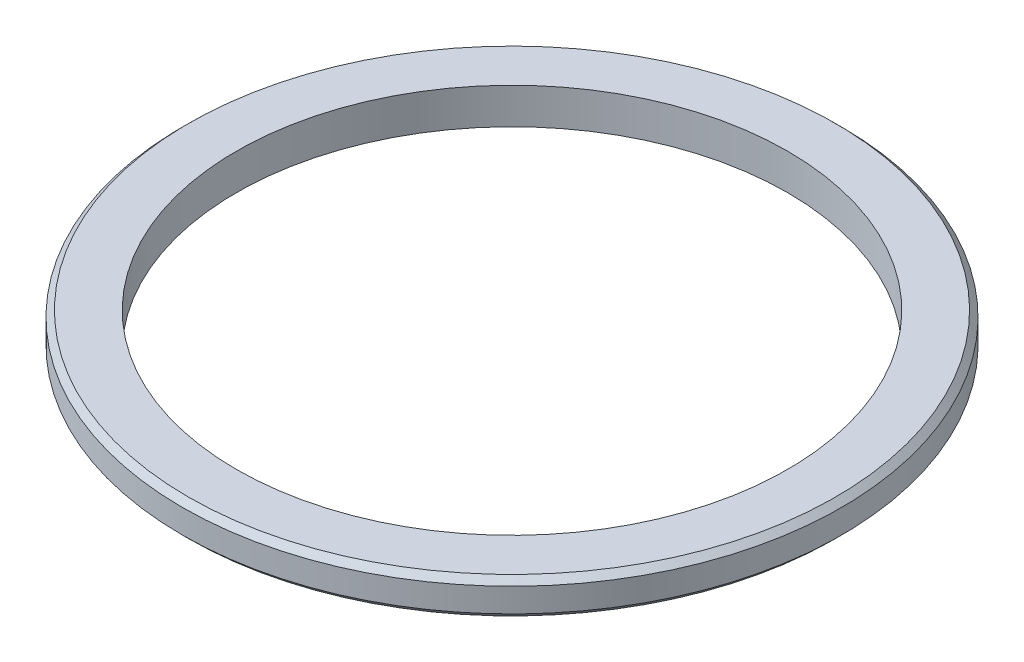
from build123d import *

# Parameters (mm, degrees)
SKETCH1_R           = 27.5
SKETCH1_R_2         = 23
BOSS_EXTRUDE1_DEPTH = 3
CHAMFER1_SIZE       = 0.5


with BuildPart() as part:
    # Sketch1 → Boss-Extrude1 (new body)
    with BuildSketch(Plane(origin=(0, 0, 0), x_dir=(1, 0, 0), z_dir=(0, 1, 0))):
        with Locations(Location((0, 0, 0), (0, 0, 270))):
            Circle(SKETCH1_R)
        with Locations(Location((0, 0, 0), (0, 0, 270))):
            Circle(SKETCH1_R_2, mode=Mode.SUBTRACT)
    extrude(amount=BOSS_EXTRUDE1_DEPTH)

    # Chamfer1
    chamfer1_edges = [part.edges().sort_by_distance(p)[0] for p in [
        (0, 0, -27.5),
        (0, 3, -27.5),
    ]]
    chamfer(chamfer1_edges, length=CHAMFER1_SIZE)


solid = part.part
